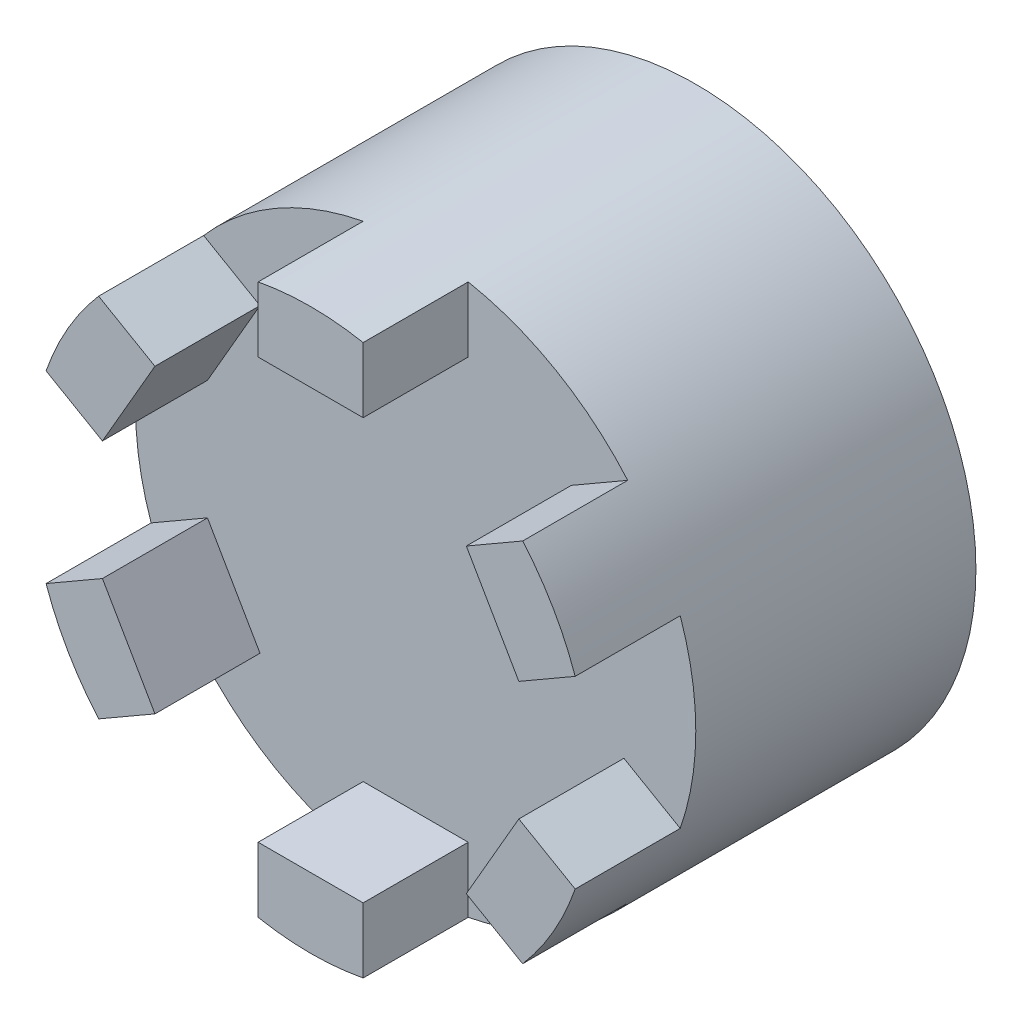
SolidWorks part; units mm, degrees
ref_plane "前视基准面" through (0, 0, 0) normal (0, 0, 1) x (1, 0, 0)
ref_plane "上视基准面" through (0, 0, 0) normal (0, 1, 0) x (1, 0, 0)
ref_plane "右视基准面" through (0, 0, 0) normal (1, 0, 0) x (0, 0, -1)
other "Configuration Table"
sketch "草图1" plane through (0, 0, 0) normal (0, 0, 1) x (1, 0, 0)
  circle A0 centre (0, 0) radius 16.5
  dimension "D1" = 33
sketch "草图2" plane through (0, 0, 0) normal (0, 0, 1) x (1, 0, 0)
  circle A0 centre (0, 0) radius 40
  dimension "D1" = 80
extrude "凸台-拉伸1" add sketch "草图2" along normal blind 40 contours A0
extrude "切除-拉伸1" cut sketch "草图1" along normal blind 30 contours A0
sketch "草图3" plane through (0, 0, 40) normal (0, 0, 1) x (1, 0, 0)
  line L0 (22.2308, 21.4952) -> (29.7308, 8.5048)
  line L2 (-7.5, 39.2906) -> (-7.5, 30)
  line L3 (-7.5, 30) -> (7.5, 30)
  line L4 (7.5, 39.2906) -> (7.5, 30)
  line L5 (30.2766, 26.1405) -> (22.2308, 21.4952)
  line L6 (37.7766, 13.1501) -> (29.7308, 8.5048)
  line L7 (29.7308, -8.5048) -> (22.2308, -21.4952)
  line L8 (37.7766, -13.1501) -> (29.7308, -8.5048)
  line L9 (30.2766, -26.1405) -> (22.2308, -21.4952)
  line L10 (7.5, -30) -> (-7.5, -30)
  line L11 (7.5, -39.2906) -> (7.5, -30)
  line L12 (-7.5, -39.2906) -> (-7.5, -30)
  line L13 (-22.2308, -21.4952) -> (-29.7308, -8.5048)
  line L14 (-30.2766, -26.1405) -> (-22.2308, -21.4952)
  line L15 (-37.7766, -13.1501) -> (-29.7308, -8.5048)
  line L16 (-29.7308, 8.5048) -> (-22.2308, 21.4952)
  line L17 (-37.7766, 13.1501) -> (-29.7308, 8.5048)
  line L18 (-30.2766, 26.1405) -> (-22.2308, 21.4952)
  arc A0 (37.7766, 13.1501) -> (30.2766, 26.1405) centre (0, 0) ccw
  circle A1 centre (0, 0) radius 40
  arc A2 (7.5, 39.2906) -> (-7.5, 39.2906) centre (0, 0) ccw
  arc A3 (30.2766, -26.1405) -> (37.7766, -13.1501) centre (0, 0) ccw
  arc A4 (-7.5, -39.2906) -> (7.5, -39.2906) centre (0, 0) ccw
  arc A5 (-37.7766, -13.1501) -> (-30.2766, -26.1405) centre (0, 0) ccw
  arc A6 (-30.2766, 26.1405) -> (-37.7766, 13.1501) centre (0, 0) ccw
  point P7 (0, 30)
  dimension "D2" = 15
  dimension "D3" = 30
  dimension "D1" = 0
  dimension "D4" = 6
extrude "凸台-拉伸2" add sketch "草图3" along normal blind 15
sketch "草图4" plane through (0, 0, 0) normal (0, 0, -1) x (-1, 0, 0)
  line L1 (-6, 19) -> (6, 19)
  line L2 (-6, 19) -> (-6, 11.4714)
  line L3 (-6, 11.4714) -> (6, 11.4714)
  line L4 (6, 19) -> (6, 11.4714)
  point P4 (0, 11.4714)
  dimension "D1" = 12
  dimension "D2" = 19
extrude "切除-拉伸2" cut sketch "草图4" against normal blind 30 contours L4 L3 L2 L1
